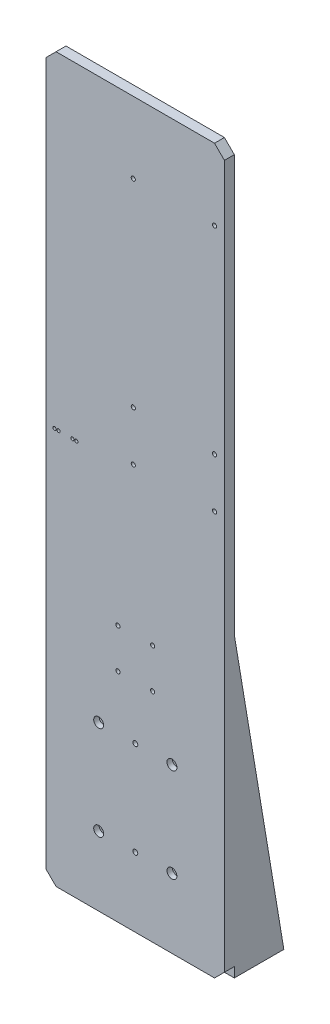
SolidWorks part; units mm, degrees
ref_plane "前视基准面" through (0, 0, 0) normal (0, 0, 1) x (1, 0, 0)
ref_plane "上视基准面" through (0, 0, 0) normal (0, 1, 0) x (1, 0, 0)
ref_plane "右视基准面" through (0, 0, 0) normal (1, 0, 0) x (0, 0, -1)
sketch "草图1" plane through (0, 0, 0) normal (0, 0, 1) x (1, 0, 0)
  line L1 (-90, 365) -> (90, 365)
  line L2 (-90, 365) -> (-90, -365)
  line L3 (-90, -365) -> (90, -365)
  line L4 (90, 365) -> (90, -365)
  line L5 (-90, 365) -> (90, -365) construction
  line L6 (-90, -365) -> (90, 365) construction
  point P0 (0, 0)
  dimension "D1" = 180
  dimension "D2" = 730
extrude "凸台-拉伸1" add sketch "草图1" along normal blind 10
hole_wizard "M5 六角凹头螺钉的柱形沉头孔1" positions "草图2" profile "草图3" counterbore size "M5" standard "ISO" end condition through all
sketch "草图2" plane through (0, 0, 10) normal (0, 0, 1) x (1, 0, 0)
  circle A4 centre (37, -295) radius 2.1 construction
  circle A5 centre (-37, -295) radius 2.1 construction
  circle A6 centre (-37, -200) radius 2.1 construction
  circle A7 centre (37, -200) radius 2.1 construction
  point P0 (-37, -200)
  point P2 (37, -200)
  point P4 (-37, -295)
  point P6 (37, -295)
sketch "草图3" plane through (-37, -200, 10) normal (1, 0, 0) x (0, -1, 0)
  line L0 (0, 0) -> (0, 10)
  line L1 (0, 10) -> (2.75, 10)
  line L3 (2.75, 10) -> (2.75, 5.4)
  line L4 (2.75, 5.4) -> (5, 5.4)
  line L5 (5, 5.4) -> (5, 0)
  line L7 (5, 0) -> (0, 0)
  line L11 (0, -6.35) -> (0, 107.95) construction
  dimension "通孔孔直径" = 5.5
  dimension "通孔孔深度" = 10
  dimension "柱形沉头孔直径" = 10
  dimension "柱形沉头孔深度" = 5.4
hole_wizard "大小mm 暗销孔0" positions "草图4" profile "草图5" hole size "Ø5.0" standard "ISO" end condition through all
sketch "草图4" plane through (0, 0, 10) normal (0, 0, 1) x (1, 0, 0)
  circle A2 centre (0, -200) radius 2.5 construction
  circle A3 centre (0, -295) radius 2.5 construction
  point P0 (0, -200)
  point P2 (0, -295)
sketch "草图5" plane through (0, -200, 10) normal (1, 0, 0) x (0, -1, 0)
  line L0 (0, 0) -> (0, 10)
  line L1 (0, 10) -> (2.5, 10)
  line L2 (2.5, 10) -> (2.5, 0)
  line L5 (2.5, 0) -> (0, 0)
  line L11 (0, -6.35) -> (0, 107.95) construction
  dimension "通孔孔直径" = 5
  dimension "通孔孔深度" = 10
chamfer "倒角1" distance 10 angle 45 4 edges at (90, -365, 5) (-90, -365, 5) (90, 365, 5) (-90, 365, 5)
hole_wizard "M5 螺纹孔2" positions "草图6" profile "草图7" tap size "M5" standard "ISO" end condition through all
sketch "草图6" plane through (0, 0, 10) normal (0, 0, 1) x (1, 0, 0)
  point P0 (80, 293)
  point P3 (-2, 293)
  point P6 (80, 93)
  point P9 (80, 43)
  point P12 (-2, 43)
  point P15 (-2, 93)
sketch "草图7" plane through (80, 293, 10) normal (1, 0, 0) x (0, -1, 0)
  line L0 (0, 0) -> (0, 10)
  line L1 (0, 10) -> (2.1, 10)
  line L2 (2.1, 10) -> (2.1, 0)
  line L5 (2.1, 0) -> (0, 0)
  line L11 (0, -6.35) -> (0, 107.95) construction
  dimension "通孔螺纹孔钻头直径" = 4.2
  dimension "通孔螺纹孔钻头深度" = 10
cosmetic thread "孔螺蚊线5" parameters "D2"=5
cosmetic thread "孔螺蚊线6" parameters "D2"=5
cosmetic thread "孔螺蚊线7" parameters "D2"=5
cosmetic thread "孔螺蚊线8" parameters "D2"=5
cosmetic thread "孔螺蚊线19" parameters "D2"=5
cosmetic thread "孔螺蚊线20" parameters "D2"=5
hole_wizard "M5 螺纹孔3" positions "草图8" profile "草图9" tap size "M5" standard "ISO" end condition through all
sketch "草图8" plane through (0, 0, 0) normal (0, 0, -1) x (-1, 0, 0)
  line L0 (-20.25, -105.5324) -> (-14.75, -105.5324)
  line L1 (-20.25, -98.2824) -> (-20.25, -112.7824) construction
  line L2 (-14.75, -98.2824) -> (-14.75, -112.7824) construction
  line L4 (14.75, -105.5324) -> (20.25, -105.5324)
  line L5 (14.75, -98.2824) -> (14.75, -112.7824) construction
  line L6 (20.25, -98.2824) -> (20.25, -112.7824) construction
  line L8 (-20.25, -145.5324) -> (-14.75, -145.5324)
  line L9 (-20.25, -138.2824) -> (-20.25, -152.7824) construction
  line L10 (-14.75, -138.2824) -> (-14.75, -152.7824) construction
  line L12 (14.75, -145.5324) -> (20.25, -145.5324)
  line L13 (14.75, -138.2824) -> (14.75, -152.7824) construction
  line L14 (20.25, -138.2824) -> (20.25, -152.7824) construction
  point P0 (-17.5, -105.5324)
  point P2 (-17.5, -145.5324)
  point P4 (17.5, -105.5324)
  point P6 (17.5, -145.5324)
sketch "草图9" plane through (17.5, -105.5324, 0) normal (1, 0, 0) x (0, 1, 0)
  line L0 (0, 0) -> (0, 10)
  line L1 (0, 10) -> (2.1, 10)
  line L2 (2.1, 10) -> (2.1, 0)
  line L5 (2.1, 0) -> (0, 0)
  line L11 (0, -6.35) -> (0, 107.95) construction
  dimension "通孔螺纹孔钻头直径" = 4.2
  dimension "通孔螺纹孔钻头深度" = 10
cosmetic thread "孔螺蚊线11" parameters "D1"=10, "D2"=5
cosmetic thread "孔螺蚊线12" parameters "D1"=10, "D2"=5
cosmetic thread "孔螺蚊线13" parameters "D1"=10, "D2"=5
cosmetic thread "孔螺蚊线14" parameters "D1"=10, "D2"=5
hole_wizard "M4 螺纹孔1" positions "草图10" profile "草图11" tap size "M4" standard "ISO" end condition through all
sketch "草图10" plane through (0, 0, 10) normal (0, 0, 1) x (1, 0, 0)
  line L0 (-81.499, 37.0429) -> (-81.499, 32.5429)
  line L1 (-80.9981, 37.0429) -> (-82, 37.0429) construction
  line L2 (-82, 32.5429) -> (-80.9981, 32.5429) construction
  line L4 (-59.4999, 37.0429) -> (-59.4999, 32.5429)
  line L5 (-59, 37.0429) -> (-59.9999, 37.0429) construction
  line L6 (-59.9999, 32.5429) -> (-59, 32.5429) construction
  point P0 (-81.499, 34.7929)
  point P2 (-59.4999, 34.7929)
  point P22 (-77.499, 34.7929)
  point P24 (-63.499, 34.7929)
  dimension "D1" = 14
  dimension "D2" = 4
sketch "草图11" plane through (-81.499, 34.7929, 10) normal (1, 0, 0) x (0, -1, 0)
  line L0 (0, 0) -> (0, 10)
  line L1 (0, 10) -> (1.65, 10)
  line L2 (1.65, 10) -> (1.65, 0)
  line L5 (1.65, 0) -> (0, 0)
  line L11 (0, -6.35) -> (0, 107.95) construction
  dimension "通孔螺纹孔钻头直径" = 3.3
  dimension "通孔螺纹孔钻头深度" = 10
cosmetic thread "孔螺蚊线15" parameters "D2"=4
cosmetic thread "孔螺蚊线16" parameters "D2"=4
cosmetic thread "孔螺蚊线17" parameters "D2"=4
cosmetic thread "孔螺蚊线18" parameters "D2"=4
sketch "草图12" plane through (-90, 0, 0) normal (-1, 0, 0) x (0, 0, 1)
  line L0 (0, -65) -> (-50, -365)
  line L1 (0, 355) -> (0, -355) construction
  line L2 (-50, -365) -> (0, -365)
  line L3 (0, -65) -> (0, -365)
  line L4 (10, -365) -> (0, -365) construction
  dimension "D1" = 50
  dimension "D2" = 300
extrude "凸台-拉伸2" add sketch "草图12" against normal blind 10
mirror "镜向1" about plane through (0, 0, 0) normal (1, 0, 0) of "凸台-拉伸2"
